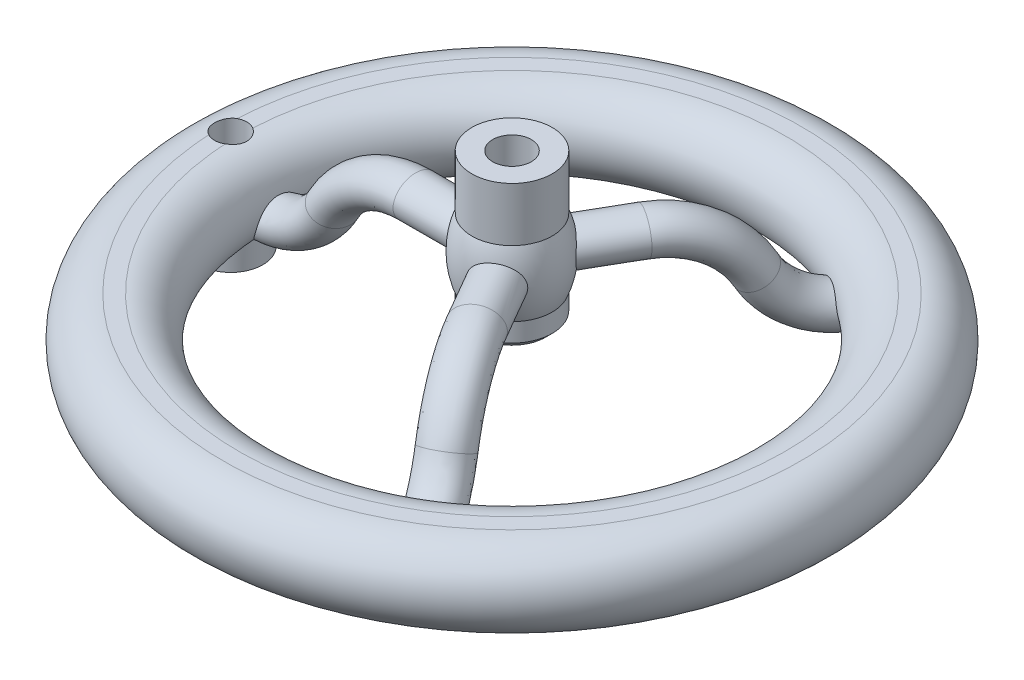
from build123d import *

# Parameters (mm, degrees)
SKETCH2_R                = 6
CUT_EXTRUDE1_DEPTH       = 16.757025
BOSS_EXTRUDE1_DEPTH      = 6
BOSS_EXTRUDE1_DEPTH_BACK = 2
SKETCH4_R                = 10
SKETCH5_RX               = 7
SKETCH5_RY               = 6
CIRPATTERN1_COUNT        = 3
SKETCH7_R                = 5
CUT_EXTRUDE2_DEPTH       = 161.756804027


with BuildPart() as part:
    # Sketch1 → Revolve1 (revolve)
    with BuildSketch(Plane.XY):
        with BuildLine():
            Line((0, 27), (-12.5, 27))
            Line((-12.5, 27), (-12.5, 10.242975314))
            ThreePointArc((-12.5, 10.242975314), (-14.51837762, 0), (-12.5, -10.242975314))
            Line((-12.5, -10.242975314), (-12.5, -16))
            Line((-12.5, -16), (-10.5, -18))
            Line((-10.5, -18), (0, -18))
            Line((0, -18), (0, 27))
        make_face()
    revolve(axis=Axis((0, 27, 0), (0, -1, 0)))

    # Sketch2 → Cut-Extrude1 (cut)
    with BuildSketch(Plane(origin=(0, 27, 0), x_dir=(1, 0, 0), z_dir=(0, 1, 0))):
        with Locations(Location((0, 0, 0), (0, 0, 180))):
            Circle(SKETCH2_R)
    extrude(amount=-CUT_EXTRUDE1_DEPTH, mode=Mode.SUBTRACT)



with BuildPart() as body_2:
    # Sketch3 → Revolve2 (revolve)
    with BuildSketch(Plane.XY, mode=Mode.PRIVATE) as revolve2_sk:
        with BuildLine():
            Line((-90, -11.5), (-85, -11.5))
            ThreePointArc((-85, -11.5), (-72.5, -24), (-85, -36.5))
            Line((-85, -36.5), (-90, -36.5))
            ThreePointArc((-90, -36.5), (-102.5, -24), (-90, -11.5))
        make_face()
    revolve(revolve2_sk.sketch.rotate(Axis((0, 0, 0), (0, -1, 0)), 270), axis=Axis((0, 0, 0), (0, -1, 0)))

    # Sketch4 → Boss-Extrude1 (add, two sides: drawn at the far end of the back side and taken through both)
    with BuildSketch(Plane.XZ.offset(36.5).offset(-BOSS_EXTRUDE1_DEPTH_BACK)):
        with Locations(Location((-87.5, 0, 0), (0, 0, 270))):
            Circle(SKETCH4_R)
    extrude(amount=BOSS_EXTRUDE1_DEPTH + BOSS_EXTRUDE1_DEPTH_BACK)


with BuildPart() as part_1:
    add(part.part)

    add(body_2.part)  # Sweep1 merges body 2
    # Sweep1: sweep along a path in Sketch6
    with BuildLine(Plane.XY) as sweep1_path:
        Line((0, 0), (-30, 0))
        ThreePointArc((-30, 0), (-44.870118242, -4.102618944), (-55.532896568, -15.249683899))
        ThreePointArc((-55.532896568, -15.249683899), (-70.714504867, -27.121103953), (-89.732142857, -24))
    # Sketch5 → Sweep1 (sweep)
    with BuildSketch(Plane(origin=(0, 0, 0), x_dir=(0, 0, -1), z_dir=(1, 0, 0))):
        with Locations(Location((0, 0), (0, 0, -180))):
            Ellipse(SKETCH5_RX, SKETCH5_RY)
    sweep1 = sweep(path=sweep1_path.line)

    # CirPattern1: Sweep1 ×3 about axis
    cirpattern1_axis = Axis((0, 0, 0), (0, -1, 0))
    for i in range(1, CIRPATTERN1_COUNT):
        add(sweep1.rotate(cirpattern1_axis, i * 360 / CIRPATTERN1_COUNT))

    # Sketch7 → Cut-Extrude2 (cut, through all)
    with BuildSketch(Plane.XZ.offset(42.5)):
        with Locations(Location((-87.5, 0, 0), (0, 0, 270))):
            Circle(SKETCH7_R)
    extrude(amount=-CUT_EXTRUDE2_DEPTH, mode=Mode.SUBTRACT)


solid = part_1.part
